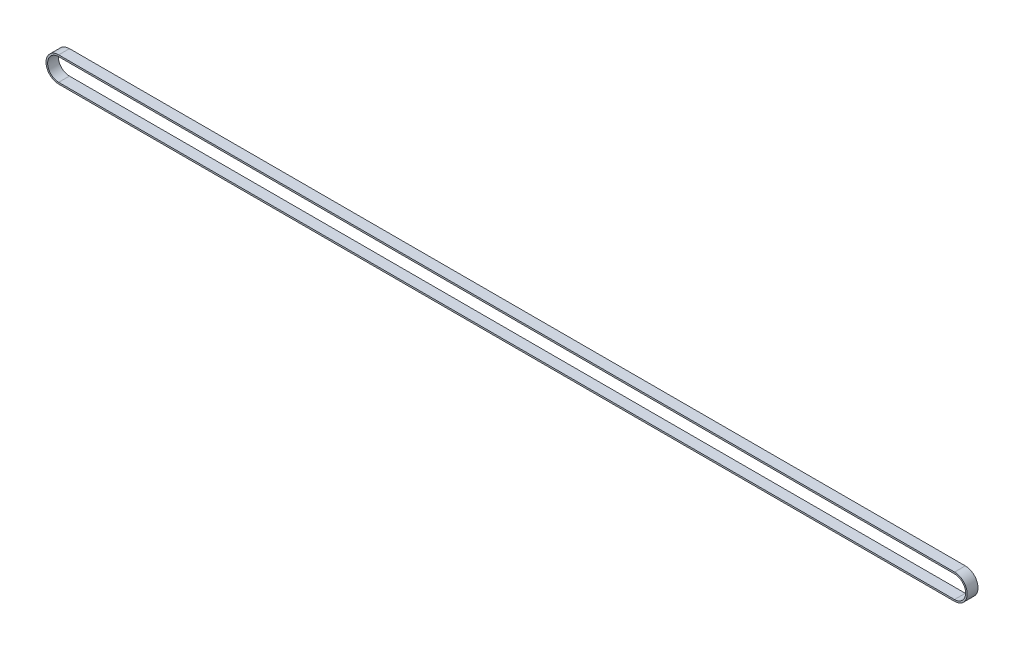
SolidWorks part; units mm, degrees
ref_plane "前视" through (0, 0, 0) normal (0, 0, 1) x (1, 0, 0)
ref_plane "上视" through (0, 0, 0) normal (0, 1, 0) x (1, 0, 0)
ref_plane "右视" through (0, 0, 0) normal (1, 0, 0) x (0, 0, -1)
sketch "草图1" plane through (0, 0, 0) normal (0, 0, 1) x (1, 0, 0)
  line L0 (-1246.5, 0) -> (1246.5, 0) construction
  line L1 (-1246.5, 31.83) -> (1246.5, 31.83)
  line L2 (-1246.5, -31.83) -> (1246.5, -31.83)
  arc A0 (-1246.5, 31.83) -> (-1246.5, -31.83) centre (-1246.5, 0) ccw
  arc A1 (1246.5, -31.83) -> (1246.5, 31.83) centre (1246.5, 0) ccw
  point P3 (0, 0)
  dimension "D1" = 63.66
  dimension "D2" = 2493
extrude "拉伸-薄壁1" add sketch "草图1" along normal blind 30 thin thin type two direction wall 3.5 second wall 1
